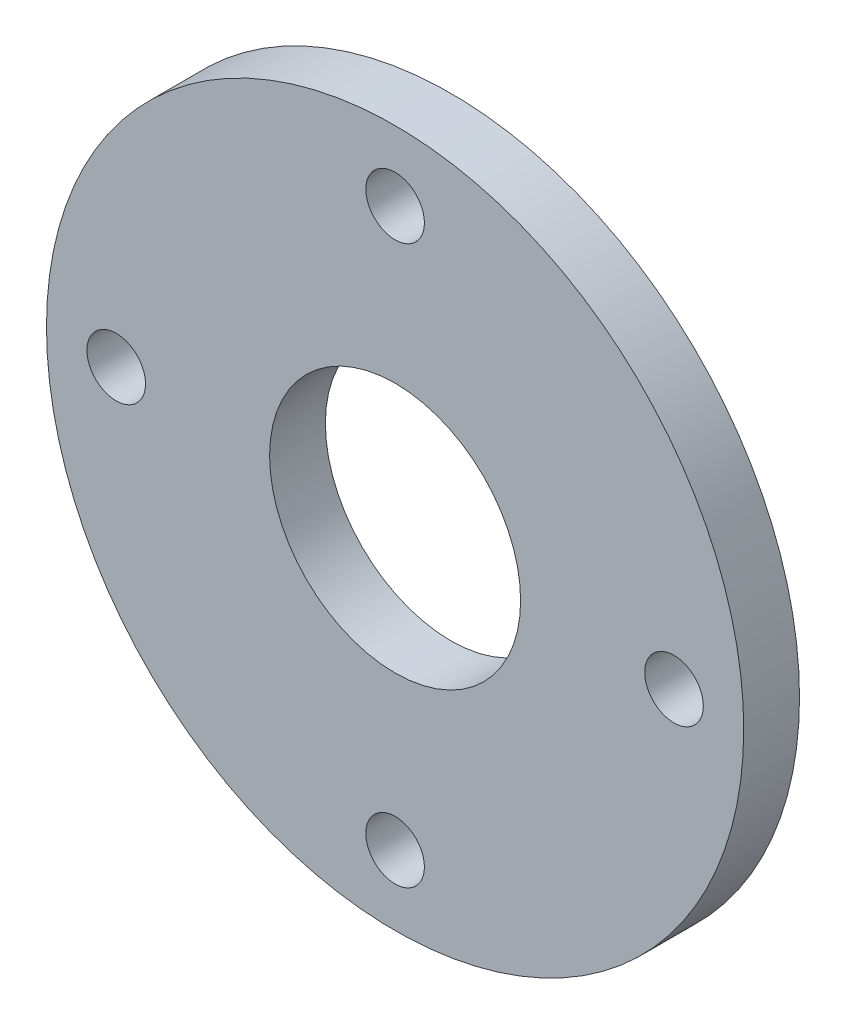
from build123d import *

# Parameters (mm, degrees)
SKETCH1_R           = 25
SKETCH1_R_2         = 9
SKETCH1_R_3         = 2.1
BOSS_EXTRUDE1_DEPTH = 4


with BuildPart() as part:
    # Sketch1 → Boss-Extrude1 (new body)
    with BuildSketch(Plane.XY):
        Circle(SKETCH1_R)
        Circle(SKETCH1_R_2, mode=Mode.SUBTRACT)
        with Locations((0, 20)):
            Circle(SKETCH1_R_3, mode=Mode.SUBTRACT)
        with Locations((-20, 0)):
            Circle(SKETCH1_R_3, mode=Mode.SUBTRACT)
        with Locations((20, 0)):
            Circle(SKETCH1_R_3, mode=Mode.SUBTRACT)
        with Locations((0, -20)):
            Circle(SKETCH1_R_3, mode=Mode.SUBTRACT)
    extrude(amount=BOSS_EXTRUDE1_DEPTH)


solid = part.part
